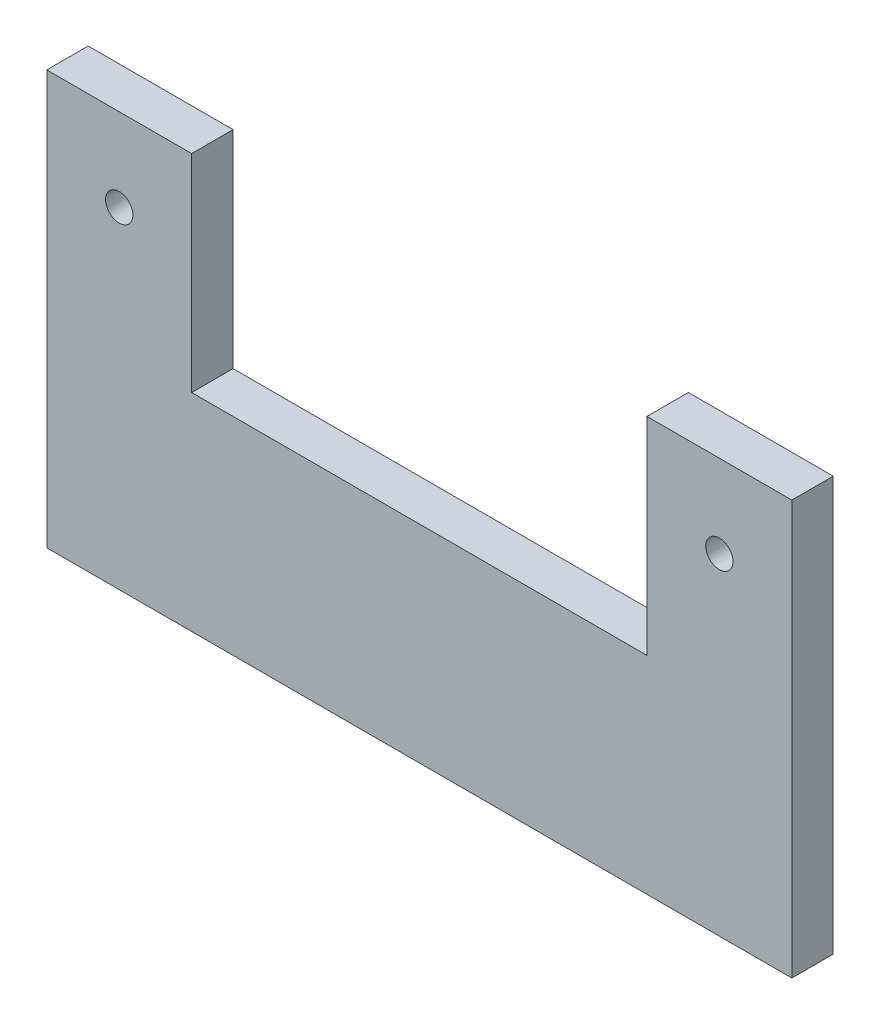
SolidWorks part; units mm, degrees
material "6061 合金"
ref_plane "前视基准面" through (0, 0, 0) normal (0, 0, 1) x (1, 0, 0)
ref_plane "上视基准面" through (0, 0, 0) normal (0, 1, 0) x (1, 0, 0)
ref_plane "右视基准面" through (0, 0, 0) normal (1, 0, 0) x (0, 0, -1)
sketch "草图1" plane through (0, 0, 0) normal (0, 0, 1) x (1, 0, 0)
  line L1 (90, -50) -> (-90, -50)
  line L2 (90, -50) -> (90, 50)
  line L3 (90, 50) -> (-90, 50)
  line L4 (-90, -50) -> (-90, 50)
  line L5 (90, -50) -> (-90, 50) construction
  line L6 (90, 50) -> (-90, -50) construction
  point P0 (0, 0)
  dimension "D1" = 180
  dimension "D2" = 100
extrude "凸台-拉伸1" add sketch "草图1" along normal blind 10
sketch "草图2" plane through (0, 0, 10) normal (0, 0, 1) x (1, 0, 0)
  line L0 (90, 50) -> (-90, 50) construction
  line L1 (55, 100) -> (-55, 100)
  line L2 (55, 100) -> (55, 0)
  line L3 (55, 0) -> (-55, 0)
  line L4 (-55, 100) -> (-55, 0)
  line L5 (55, 100) -> (-55, 0) construction
  line L6 (55, 0) -> (-55, 100) construction
  line L7 (-90, 50) -> (-90, -50) construction
  point P0 (0, 50)
  dimension "D1" = 35
  dimension "D2" = 50
extrude "切除-拉伸1" cut sketch "草图2" against normal up to next
sketch "草图5" plane through (0, 0, 0) normal (0, 0, -1) x (-1, 0, 0)
  line L0 (-72.5, 50) -> (-72.5, 30) construction
  line L1 (-90, 50) -> (-55, 50) construction
  line L2 (-72.5, 30) -> (72.5, 30) construction
  line L3 (72.5, 30) -> (72.5, 50) construction
  line L4 (55, 50) -> (90, 50) construction
  point P0 (-72.5, 30)
  point P2 (72.5, 30)
  dimension "D1" = 20
hole_wizard "M6 间隙孔1" positions "草图5" profile "草图4" hole size "M6" standard "GB" end condition up to next
sketch "草图4" plane through (72.5, 30, 0) normal (1, 0, 0) x (0, 1, 0)
  line L0 (0, 0) -> (0, 10)
  line L1 (0, 10) -> (3.3, 10)
  line L2 (3.3, 10) -> (3.3, 0)
  line L5 (3.3, 0) -> (0, 0)
  line L11 (0, -6.35) -> (0, 107.95) construction
  dimension "通孔孔直径" = 6.6
  dimension "通孔孔深度" = 10
